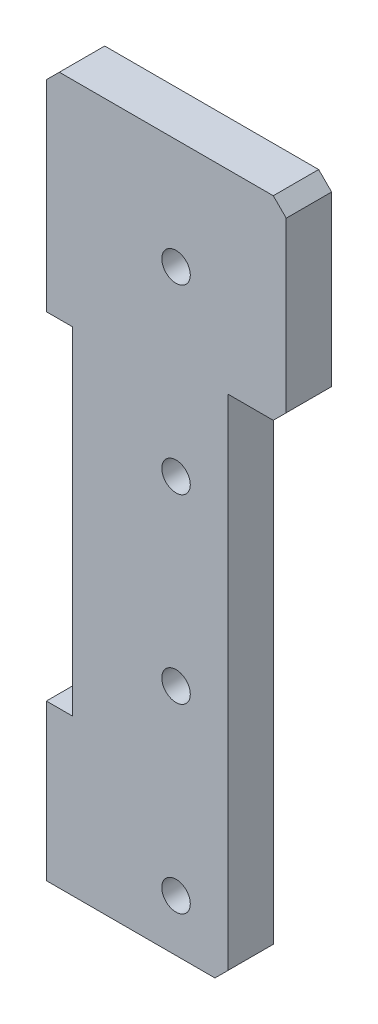
from build123d import *

# Parameters (mm, degrees)
BOSS_EXTRUDE1_DEPTH     = 35
CHAMFER1_SIZE           = 10
CUT_EXTRUDE1_DEPTH      = 577.606451577
CUT_EXTRUDE1_DEPTH_BACK = 577.606451577
SKETCH2_R               = 11


with BuildPart() as part:
    # Sketch1 → Boss-Extrude1 (new body)
    with BuildSketch(Plane.XY):
        Polygon((185, -150), (185, 0), (0, 0), (0, -165), (20, -165), (20, -425), (0, -425), (0, -545), (140, -545), (140, -150), align=None)
    extrude(amount=BOSS_EXTRUDE1_DEPTH)

    # Chamfer1
    chamfer1_edges = [part.edges().sort_by_distance(p)[0] for p in [
        (140, -545, 17.5),
        (0, 0, 17.5),
        (185, 0, 17.5),
        (185, -150, 17.5),
    ]]
    chamfer(chamfer1_edges, length=CHAMFER1_SIZE)

    # Sketch2 → Cut-Extrude1 (cut, two sides: drawn at the far end of the back side and taken through both)
    with BuildSketch(Plane.XY.offset(35).offset(-CUT_EXTRUDE1_DEPTH_BACK)):
        with Locations((100, -85)):
            Circle(SKETCH2_R)
        with Locations((100, -225)):
            Circle(SKETCH2_R)
        with Locations((100, -365)):
            Circle(SKETCH2_R)
        with Locations((100, -505)):
            Circle(SKETCH2_R)
    extrude(amount=CUT_EXTRUDE1_DEPTH + CUT_EXTRUDE1_DEPTH_BACK, mode=Mode.SUBTRACT)


solid = part.part
